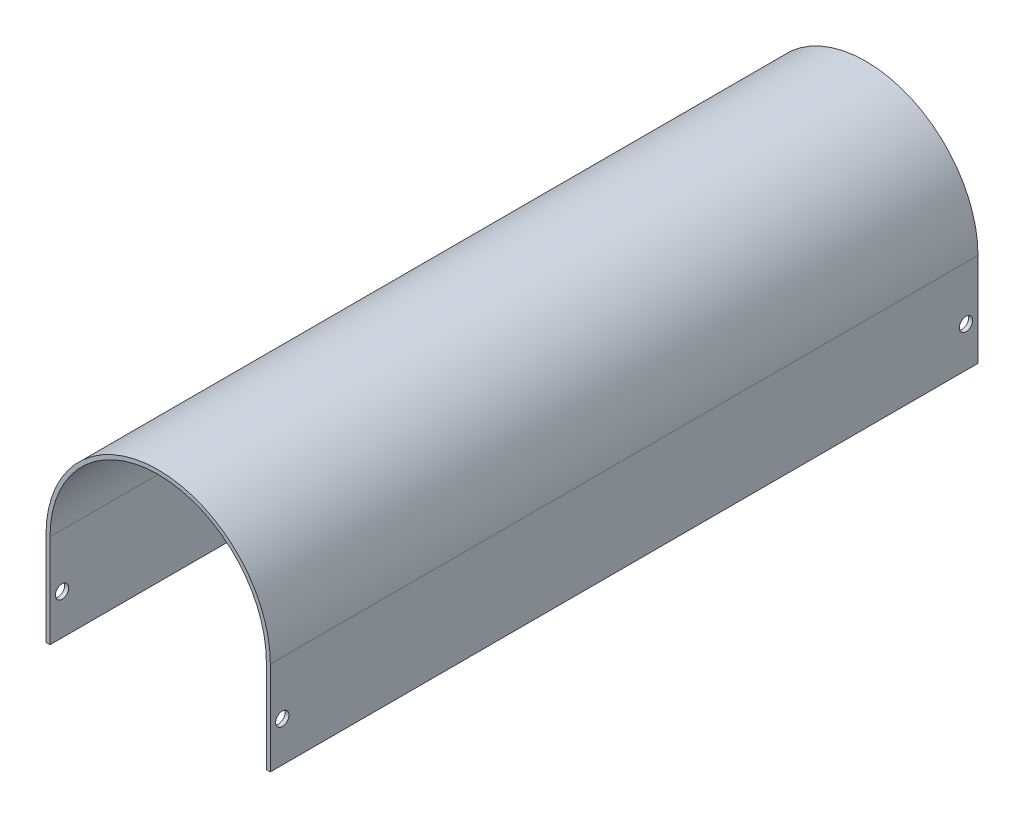
SolidWorks part; units mm, degrees
material "普通碳钢"
ref_plane "前视基准面" through (0, 0, 0) normal (0, 0, 1) x (1, 0, 0)
ref_plane "上视基准面" through (0, 0, 0) normal (0, 1, 0) x (1, 0, 0)
ref_plane "右视基准面" through (0, 0, 0) normal (1, 0, 0) x (0, 0, -1)
sketch "草图1" plane through (0, 0, 0) normal (0, 0, 1) x (1, 0, 0)
  line L0 (-20.5822, 0) -> (-19.0822, 0)
  line L1 (-54.0327, 35) -> (96.8683, 35) construction
  line L2 (0, -25.3936) -> (0, 125.9735) construction
  line L3 (63.4178, 35) -> (63.4178, 0)
  line L4 (61.9178, 35) -> (61.9178, 0)
  line L5 (-19.0822, 35) -> (-19.0822, 0)
  line L6 (-20.5822, 35) -> (-20.5822, 0)
  line L7 (61.9178, 0) -> (63.4178, 0)
  line L8 (-54.0327, 0) -> (96.8683, 0) construction
  arc A0 (63.4178, 35) -> (-20.5822, 35) centre (21.4178, 35) ccw
  arc A1 (61.9178, 35) -> (-19.0822, 35) centre (21.4178, 35) ccw
  dimension "D2" = 84
  dimension "D3" = 81
  dimension "D1" = 35
extrude "凸台-拉伸1" add sketch "草图1" along normal blind 265
sketch "草图2" plane through (63.4178, 0, 0) normal (1, 0, 0) x (0, 0, -1)
  line L1 (-132.5, 106.6246) -> (-132.5, -73.7557) construction
  line L2 (-265, 15) -> (0, 15)
  line L3 (-265, 15) -> (0, 15) construction
  line L4 (-260.5, 106.6246) -> (-260.5, -73.7557) construction
  line L5 (-4.5, 106.6246) -> (-4.5, -73.7557) construction
  circle A0 centre (-260.5, 15) radius 2.5
  circle A1 centre (-4.5, 15) radius 2.5
  dimension "D4" = 5
  dimension "D5" = 5
  dimension "D1" = 15
  dimension "D2" = 128
  dimension "D3" = 128
extrude "切除-拉伸1" cut sketch "草图2" against normal through all
